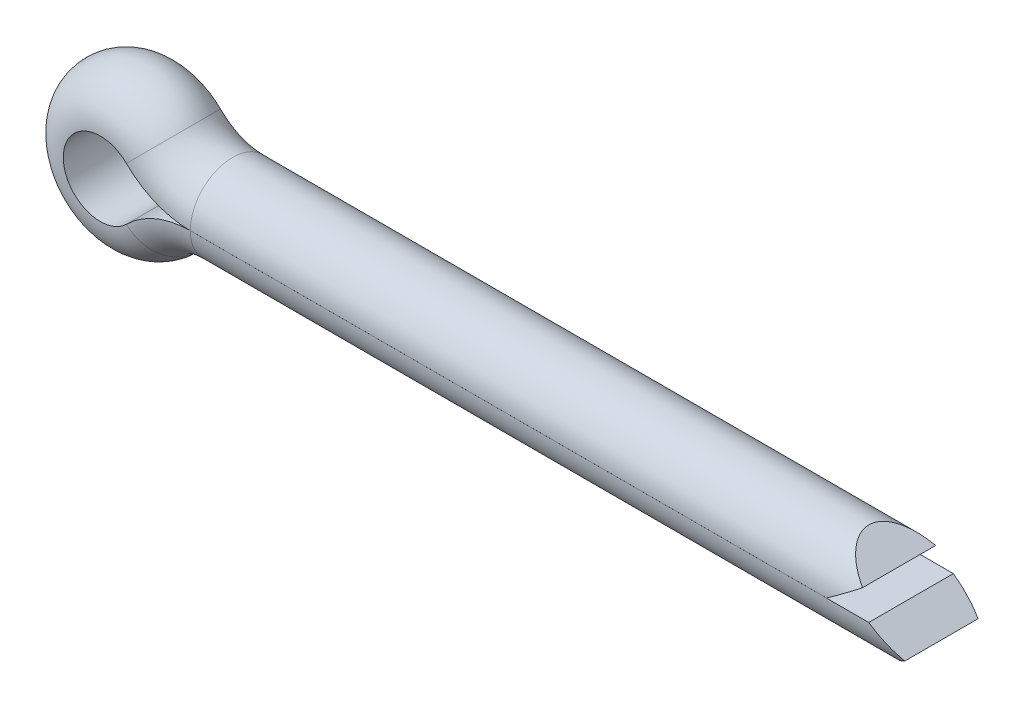
SolidWorks part; units mm, degrees
material "Q215"
ref_plane "Front" through (0, 0, 0) normal (0, 0, 1) x (1, 0, 0)
ref_plane "Top" through (0, 0, 0) normal (0, 1, 0) x (1, 0, 0)
ref_plane "Right" through (0, 0, 0) normal (1, 0, 0) x (0, 0, -1)
sketch "草图2" plane through (0, 0, 0) normal (0, 0, 1) x (1, 0, 0)
  line L0 (63, 4) -> (0, 4)
  line L1 (0, -4) -> (67, -4)
  line L2 (0, 0) -> (49.7718, 0) construction
  line L3 (0, 0) -> (0, 16.5256) construction
  line L4 (-16, 0) -> (-16, 14.2137) construction
  arc A0 (0, 4) -> (-3.2189, 5.3254) centre (0, 8.5714) cw
  arc A1 (-3.2189, 5.3254) -> (-3.2189, -5.3254) centre (-8.5, 0) ccw
  arc A2 (-3.2189, -5.3254) -> (0, -4) centre (0, -8.5714) cw
ref_plane "SectionPlane" through (63, 0, 0) normal (1, 0, 0) x (0, 0, -1)
sketch "草图1" plane through (63, 0, 0) normal (1, 0, 0) x (0, 0, -1)
  line L1 (-4, 0.002) -> (4, 0.002)
  arc A0 (4, 0.002) -> (-4, 0.002) centre (0, 0) ccw
sweep "Body" add profiles "草图1" path "草图2"
sketch "草图3" plane through (0, 0, 0) normal (0, 0, 1) x (1, 0, 0)
  line L0 (0, 0) -> (0, 16.2682) construction
  line L1 (0, 0) -> (75.9079, 0) construction
  line L2 (0, 0) -> (67, 0) construction
  line L3 (63, 2.001) -> (60.1394, 4.01)
  line L4 (63, 0.002) -> (63, 4) construction
  line L6 (63, 2.001) -> (60.1338, 0)
  line L7 (67, -2.001) -> (64.1338, 0)
  line L8 (67, -4) -> (67, -0.002) construction
  line L9 (67, -2.001) -> (64.1394, -4.01)
  line L10 (64.1338, 0) -> (60.1338, 0)
  line L11 (60.1394, 4.01) -> (67.01, 4.01)
  line L12 (67.01, 4.01) -> (67.01, -4.01)
  line L13 (67.01, -4.01) -> (64.1394, -4.01)
  line L14 (63, 4) -> (0, 4) construction
  dimension "D1" = 0.01
  dimension "D2" = 0.01
  dimension "D3" = 70
  dimension "D4" = 70
extrude "ConeCut" cut sketch "草图3" against normal through all and the other way through all
equation "' \"Diameter@草图2\" = 9.5"
equation "' \"c@草图2\" = 19"
equation "' \"b@草图2\" = 20"
equation "' \"a@草图2\" = 6.3"
equation "' \"l@草图2\" = 45"
equation "' \"Diameter@草图2\" = 1"
equation "' \"c@草图2\" = 2"
equation "' \"b@草图2\" = 3"
equation "' \"a@草图2\" = 2.5"
equation "' \"l@草图2\" = 8"
equation "' \"Diameter@草图2\" = 0.5"
equation "' \"c@草图2\" = 1"
equation "' \"b@草图2\" = 2"
equation "' \"a@草图2\" = 1.6"
equation "' \"l@草图2\" = 4"
equation "\"Diameter@草图1\" = \"Diameter@草图2\""
equation "\"Length@SectionPlane\" = \"l@草图2\""
